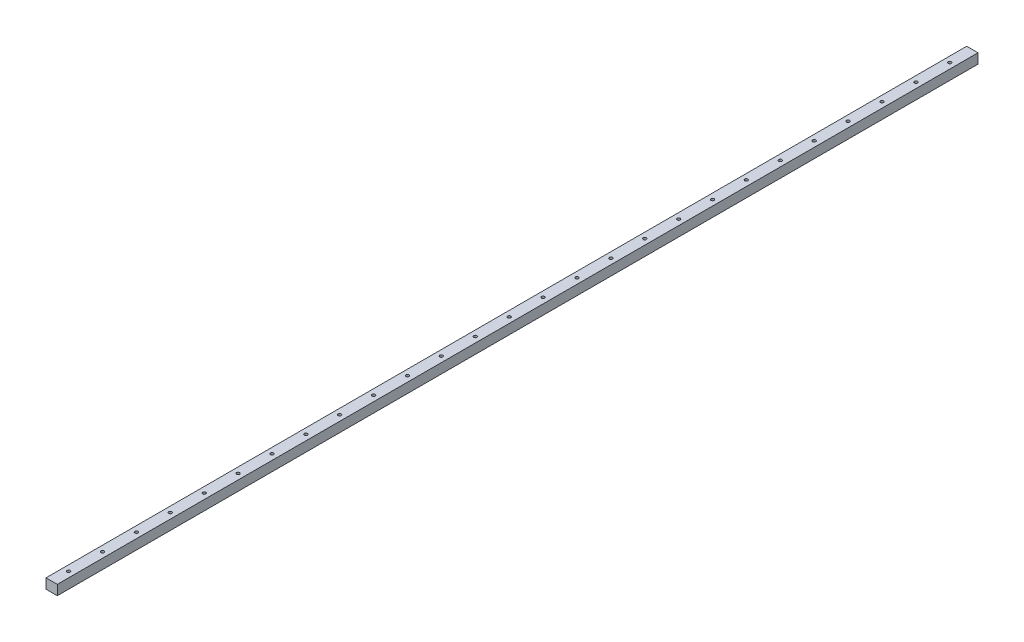
SolidWorks part; units mm, degrees
ref_plane "前视基准面" through (0, 0, 0) normal (0, 0, 1) x (1, 0, 0)
ref_plane "上视基准面" through (0, 0, 0) normal (0, 1, 0) x (1, 0, 0)
ref_plane "右视基准面" through (0, 0, 0) normal (1, 0, 0) x (0, 0, -1)
sketch "草图1" plane through (0, 0, 0) normal (0, 0, 1) x (1, 0, 0)
  line L1 (0, 0) -> (20, 0)
  line L2 (0, 0) -> (0, 17.5)
  line L3 (0, 17.5) -> (20, 17.5)
  line L4 (20, 0) -> (20, 17.5)
  dimension "D1" = 20
  dimension "D2" = 17.5
extrude "凸台-拉伸1" add sketch "草图1" along normal blind 1630
hole_wizard "打孔尺寸(%根据)内六角圆柱头螺钉的类型1" positions "草图3" profile "草图2" counterbore size "M5" standard "GB" end condition through all
sketch "草图3" plane through (0, 0, 0) normal (0, -1, 0) x (-1, 0, 0)
  line L0 (-10, -1630) -> (-10, -1466.3182) construction
  line L1 (0, -1630) -> (-20, -1630) construction
  point P0 (-10, -1600)
  dimension "D1" = 30
sketch "草图2" plane through (10, 0, 1600) normal (1, 0, 0) x (0, 0, -1)
  line L0 (0, 0) -> (0, 17.5)
  line L1 (0, 17.5) -> (2.75, 17.5)
  line L3 (2.75, 17.5) -> (2.75, 5.7)
  line L4 (2.75, 5.7) -> (5, 5.7)
  line L5 (5, 5.7) -> (5, 0)
  line L7 (5, 0) -> (0, 0)
  line L11 (0, -6.35) -> (0, 107.95) construction
  dimension "通孔孔直径" = 5.5
  dimension "通孔孔深度" = 17.5
  dimension "柱形沉头孔直径" = 10
  dimension "柱形沉头孔深度" = 5.7
pattern_linear "阵列(线性)1" count 27 spacing 60 along (0, 0, -1) of "打孔尺寸(%根据)内六角圆柱头螺钉的类型1"
